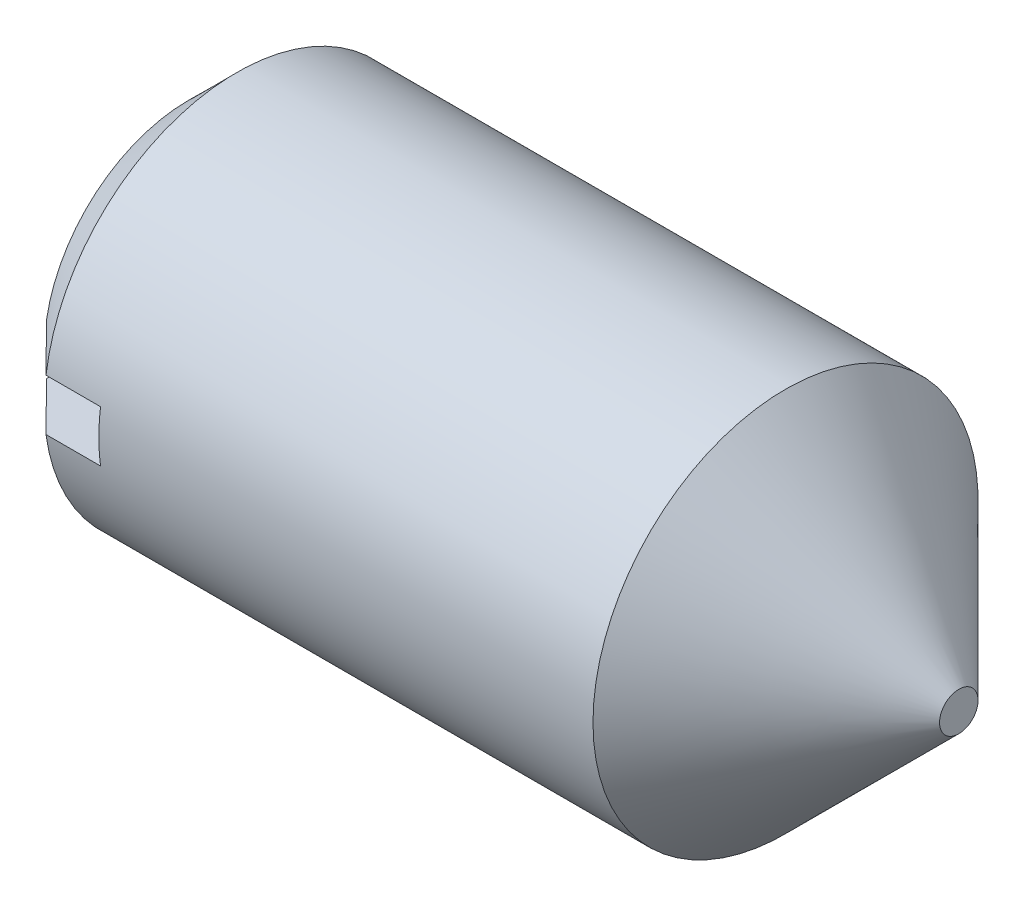
SolidWorks part; units mm, degrees
ref_plane "Front" through (0, 0, 0) normal (0, 0, 1) x (1, 0, 0)
ref_plane "Top" through (0, 0, 0) normal (0, 1, 0) x (1, 0, 0)
ref_plane "Right" through (0, 0, 0) normal (1, 0, 0) x (0, 0, -1)
other "Configuration Table"
sketch "Sketch1" plane through (0, 0, 0) normal (0, 0, 1) x (1, 0, 0)
  line L0 (0, 0) -> (6, 0)
  line L1 (6, 0) -> (6, 0.15)
  line L2 (6, 0.15) -> (4.65, 1.5)
  line L3 (4.65, 1.5) -> (0.375, 1.5)
  line L4 (0.375, 1.5) -> (0, 1.125)
  line L5 (0, 1.125) -> (0, 0)
  line L6 (-14.7741, 0) -> (12.5137, 0) construction
revolve "Base" add sketch "Sketch1" angle 360 about L6
cosmetic thread "ThreadCosmetic1" [suppressed] parameters "D2"=2.25
sketch "Sketch2" plane through (0, 0, 0) normal (0, 0, 1) x (1, 0, 0)
  line L1 (0, 0.2) -> (0.8, 0.2)
  line L2 (0, 0.2) -> (0, -0.2)
  line L3 (0, -0.2) -> (0.8, -0.2)
  line L4 (0.8, 0.2) -> (0.8, -0.2)
  line L5 (0, 1.125) -> (0, -1.125) construction
extrude "Notch" cut sketch "Sketch2" against normal through all and the other way through all
sketch "Sketch3" plane through (0, 0, 0) normal (0, 0, 1) x (1, 0, 0)
  line L0 (0.375, 1.1752) -> (0.5625, 1.5)
  line L1 (0.5625, 1.5) -> (0.5625, 1.875)
  line L2 (0.5625, 1.875) -> (0.1875, 1.875)
  line L3 (0.1875, 1.875) -> (0.1875, 1.5)
  line L4 (0.1875, 1.5) -> (0.375, 1.1752)
  line L5 (0, 0) -> (2.4208, 0) construction
  line L6 (0.375, 1.5) -> (0.375, 0.2) construction
revolve "Cut-Revolve10" [suppressed] cut sketch "Sketch3" angle 360 about L5
pattern_linear "LPattern10" [suppressed] count 20 spacing 0.9744 along (1, 0, 0)
equation "\"df@Sketch1\" = \"D2@ThreadCosmetic1\""
equation "\"m@Sketch2\" = \"n@Sketch2\" / 2"
equation "\"D1@Sketch3\" = \"d@Sketch1\""
equation "\"D2@Sketch3\" =  ( \"d@Sketch1\" - \"D2@ThreadCosmetic1\" )  / 2"
equation "\"D3@LPattern10\" = \"D2@Sketch3\" * 1.2"
equation "\"D1@LPattern10\" =  ( \"l@Sketch1\" -  ( \"d@Sketch1\" - \"df@Sketch1\" )  / 2 )  / \"D3@LPattern10\""
